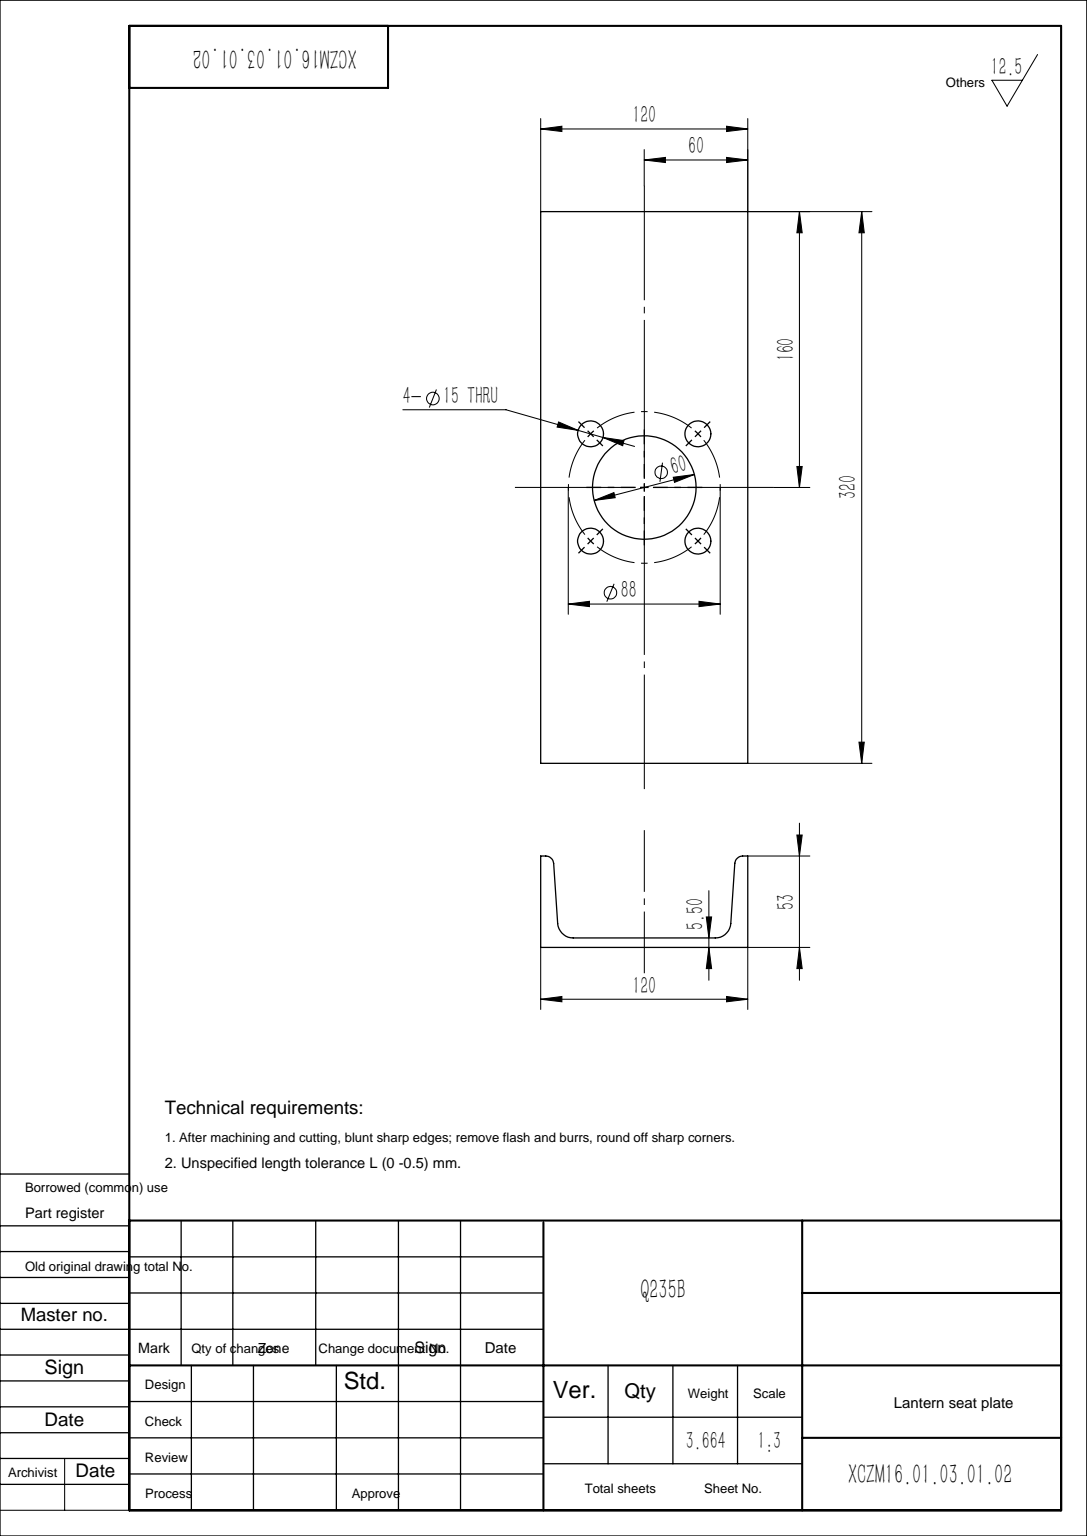
SolidWorks part; units mm, degrees
material "XRAAT"
ref_plane "前视基准面" through (0, 0, 0) normal (0, 0, 1) x (1, 0, 0)
ref_plane "上视基准面" through (0, 0, 0) normal (0, 1, 0) x (1, 0, 0)
ref_plane "右视基准面" through (0, 0, 0) normal (1, 0, 0) x (0, 0, -1)
sketch "草图1" plane through (0, 0, 0) normal (0, 0, 1) x (1, 0, 0)
  line L0 (0, 0) -> (0, 320)
  dimension "D1" = 320
other "槽钢 12(1)"
ref_plane "基准面1" through (0, 0, 0) normal (0, 1, 0) x (0, 0, 1)
sketch "Sketch1" plane through (0, 0, 0) normal (0, 1, 0) x (0, 0, 1)
  line L0 (0, 0) -> (0, -120)
  line L1 (0, -120) -> (-53, -120)
  line L2 (0, -60) -> (-5.5, -60) construction
  line L3 (-5.5, -101.1579) -> (-5.5, -18.8421)
  line L4 (-13.8856, -110.1369) -> (-48.8072, -112.5263)
  line L5 (-53, -117.0158) -> (-53, -120)
  line L6 (-5.5, -109.5632) -> (-5.5, -112.8132) construction
  line L7 (-5.5, -112.8132) -> (-53, -112.8132) construction
  line L8 (-26.5, -120) -> (-26.5, -111) construction
  line L9 (-53, -2.9842) -> (-53, 0)
  line L10 (0, 0) -> (-53, 0)
  line L11 (-13.8856, -9.8631) -> (-48.8072, -7.4737)
  arc A0 (-5.5, -101.1579) -> (-13.8856, -110.1369) centre (-14.5, -101.1579) cw
  arc A1 (-13.8856, -9.8631) -> (-5.5, -18.8421) centre (-14.5, -18.8421) cw
  arc A2 (-48.8072, -112.5263) -> (-53, -117.0158) centre (-48.5, -117.0158) ccw
  arc A3 (-53, -2.9842) -> (-48.8072, -7.4737) centre (-48.5, -2.9842) ccw
  point P2 (-26.5, 0)
  point P17 (0, 0)
  point P20 (-5.5, -10.4368)
  point P26 (-53, -7.1868)
  dimension "r" = 9
  dimension "r1" = 4.5
  dimension "h" = 120
  dimension "b" = 53
  dimension "d" = 5.5
  dimension "t" = 9
  dimension "D5" = 47.5
  dimension "D6" = 3.25
sketch "草图5" plane through (0, 0, 0) normal (0, 0, 1) x (1, 0, 0)
  line L1 (-60, 320) -> (-60, 160) construction
  line L2 (-120, 320) -> (0, 320) construction
  circle A0 centre (-60, 160) radius 30
  circle A1 centre (-91.1127, 191.1127) radius 7.5
  circle A2 centre (-60, 160) radius 44 construction
  circle A3 centre (-28.8873, 191.1127) radius 7.5
  circle A4 centre (-28.8873, 128.8873) radius 7.5
  circle A5 centre (-91.1127, 128.8873) radius 7.5
  point P17 (-60, 160)
  dimension "D2" = 60
  dimension "D3" = 15
  dimension "D4" = 88
  dimension "D1" = 160
  dimension "D5" = 4
extrude "切除-拉伸1" cut sketch "草图5" against normal blind 10
